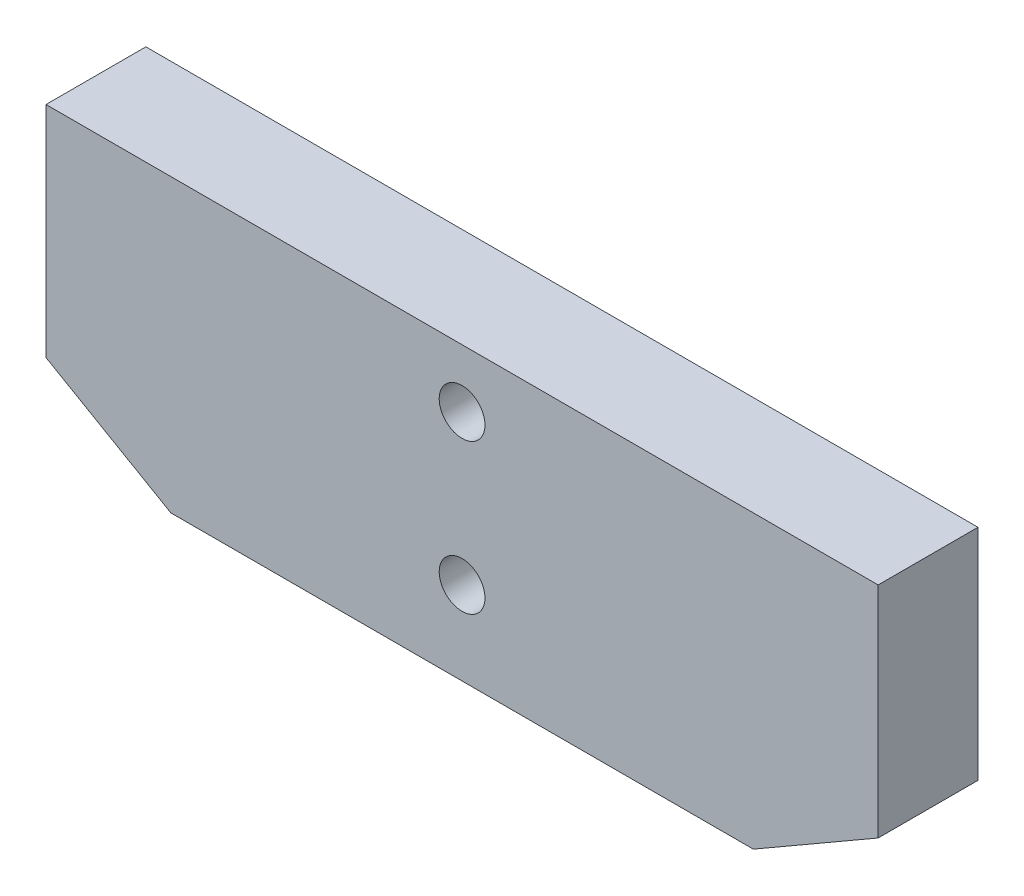
SolidWorks part; units mm, degrees
ref_plane "前视基准面" through (0, 0, 0) normal (0, 0, 1) x (1, 0, 0)
ref_plane "上视基准面" through (0, 0, 0) normal (0, 1, 0) x (1, 0, 0)
ref_plane "右视基准面" through (0, 0, 0) normal (1, 0, 0) x (0, 0, -1)
sketch "草图1" plane through (0, 0, 0) normal (0, 0, 1) x (1, 0, 0)
  line L1 (50, -17.5) -> (-50, -17.5)
  line L2 (50, -17.5) -> (50, 17.5)
  line L3 (50, 17.5) -> (-50, 17.5)
  line L4 (-50, -17.5) -> (-50, 17.5)
  line L5 (50, -17.5) -> (-50, 17.5) construction
  line L6 (50, 17.5) -> (-50, -17.5) construction
  point P0 (0, 0)
  dimension "D1" = 35
  dimension "D2" = 100
extrude "凸台-拉伸1" add sketch "草图1" along normal blind 12
chamfer "倒角1" distance 15 angle 30 2 edges at (50, -17.5, 6) (-50, -17.5, 6)
hole_wizard "打孔尺寸(%根据)内六角圆柱头螺钉的类型1" positions "草图2" profile "草图3" counterbore size "M5" standard "GB" end condition up to next
sketch "草图2" plane through (0, 0, 0) normal (0, 0, -1) x (-1, 0, 0)
  point P0 (0, 10.5)
  point P3 (0, -7.5)
sketch "草图3" plane through (0, 10.5, 0) normal (1, 0, 0) x (0, 1, 0)
  line L0 (0, 0) -> (0, 12)
  line L1 (0, 12) -> (2.75, 12)
  line L3 (2.75, 12) -> (2.75, 5.7)
  line L4 (2.75, 5.7) -> (5, 5.7)
  line L5 (5, 5.7) -> (5, 0)
  line L7 (5, 0) -> (0, 0)
  line L11 (0, -6.35) -> (0, 107.95) construction
  dimension "通孔孔直径" = 5.5
  dimension "通孔孔深度" = 12
  dimension "柱形沉头孔直径" = 10
  dimension "柱形沉头孔深度" = 5.7
